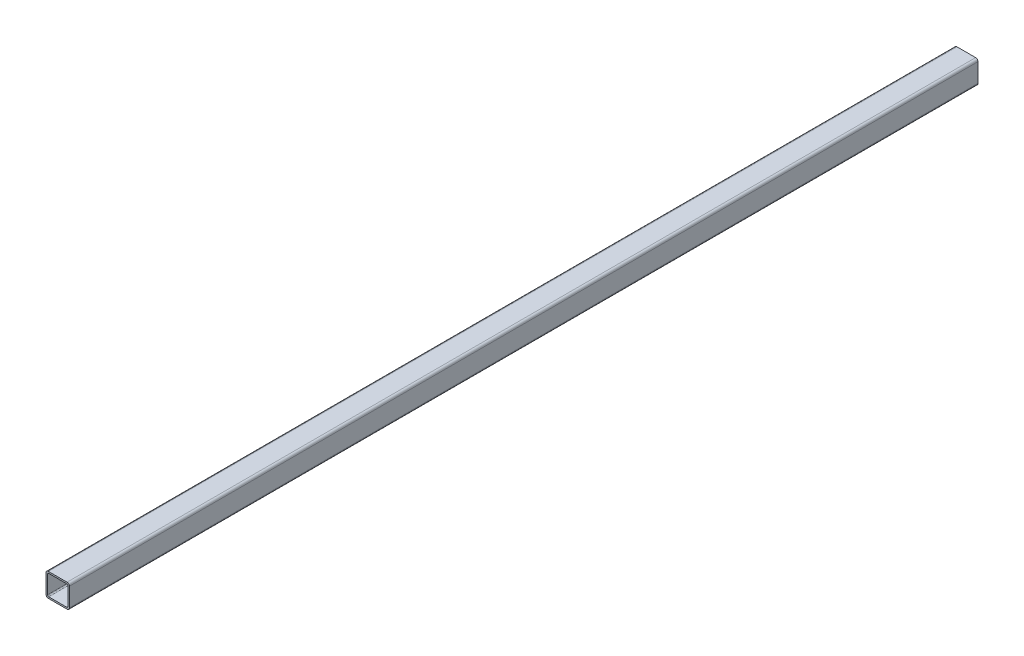
from build123d import *

# Parameters (mm, degrees)
SKETCH1_W           = 60
SKETCH1_H           = 60
SKETCH1_W_2         = 52
SKETCH1_H_2         = 52
BOSS_EXTRUDE1_DEPTH = 1165
FILLET1_R           = 6
FILLET2_R           = 3


with BuildPart() as part:
    # Sketch1 → Boss-Extrude1 (new, symmetric)
    with BuildSketch(Plane.XY):
        Rectangle(SKETCH1_W, SKETCH1_H)
        Rectangle(SKETCH1_W_2, SKETCH1_H_2, mode=Mode.SUBTRACT)
    extrude(amount=BOSS_EXTRUDE1_DEPTH, both=True)

    # Fillet1
    fillet1_edges = [part.edges().sort_by_distance(p)[0] for p in [
        (30, -30, 0),
        (-30, -30, 0),
        (-30, 30, 0),
        (30, 30, 0),
    ]]
    fillet(fillet1_edges, radius=FILLET1_R)

    # Fillet2
    fillet2_edges = [part.edges().sort_by_distance(p)[0] for p in [
        (26, -26, 0),
        (26, 26, 0),
        (-26, 26, 0),
        (-26, -26, 0),
    ]]
    fillet(fillet2_edges, radius=FILLET2_R)


solid = part.part
